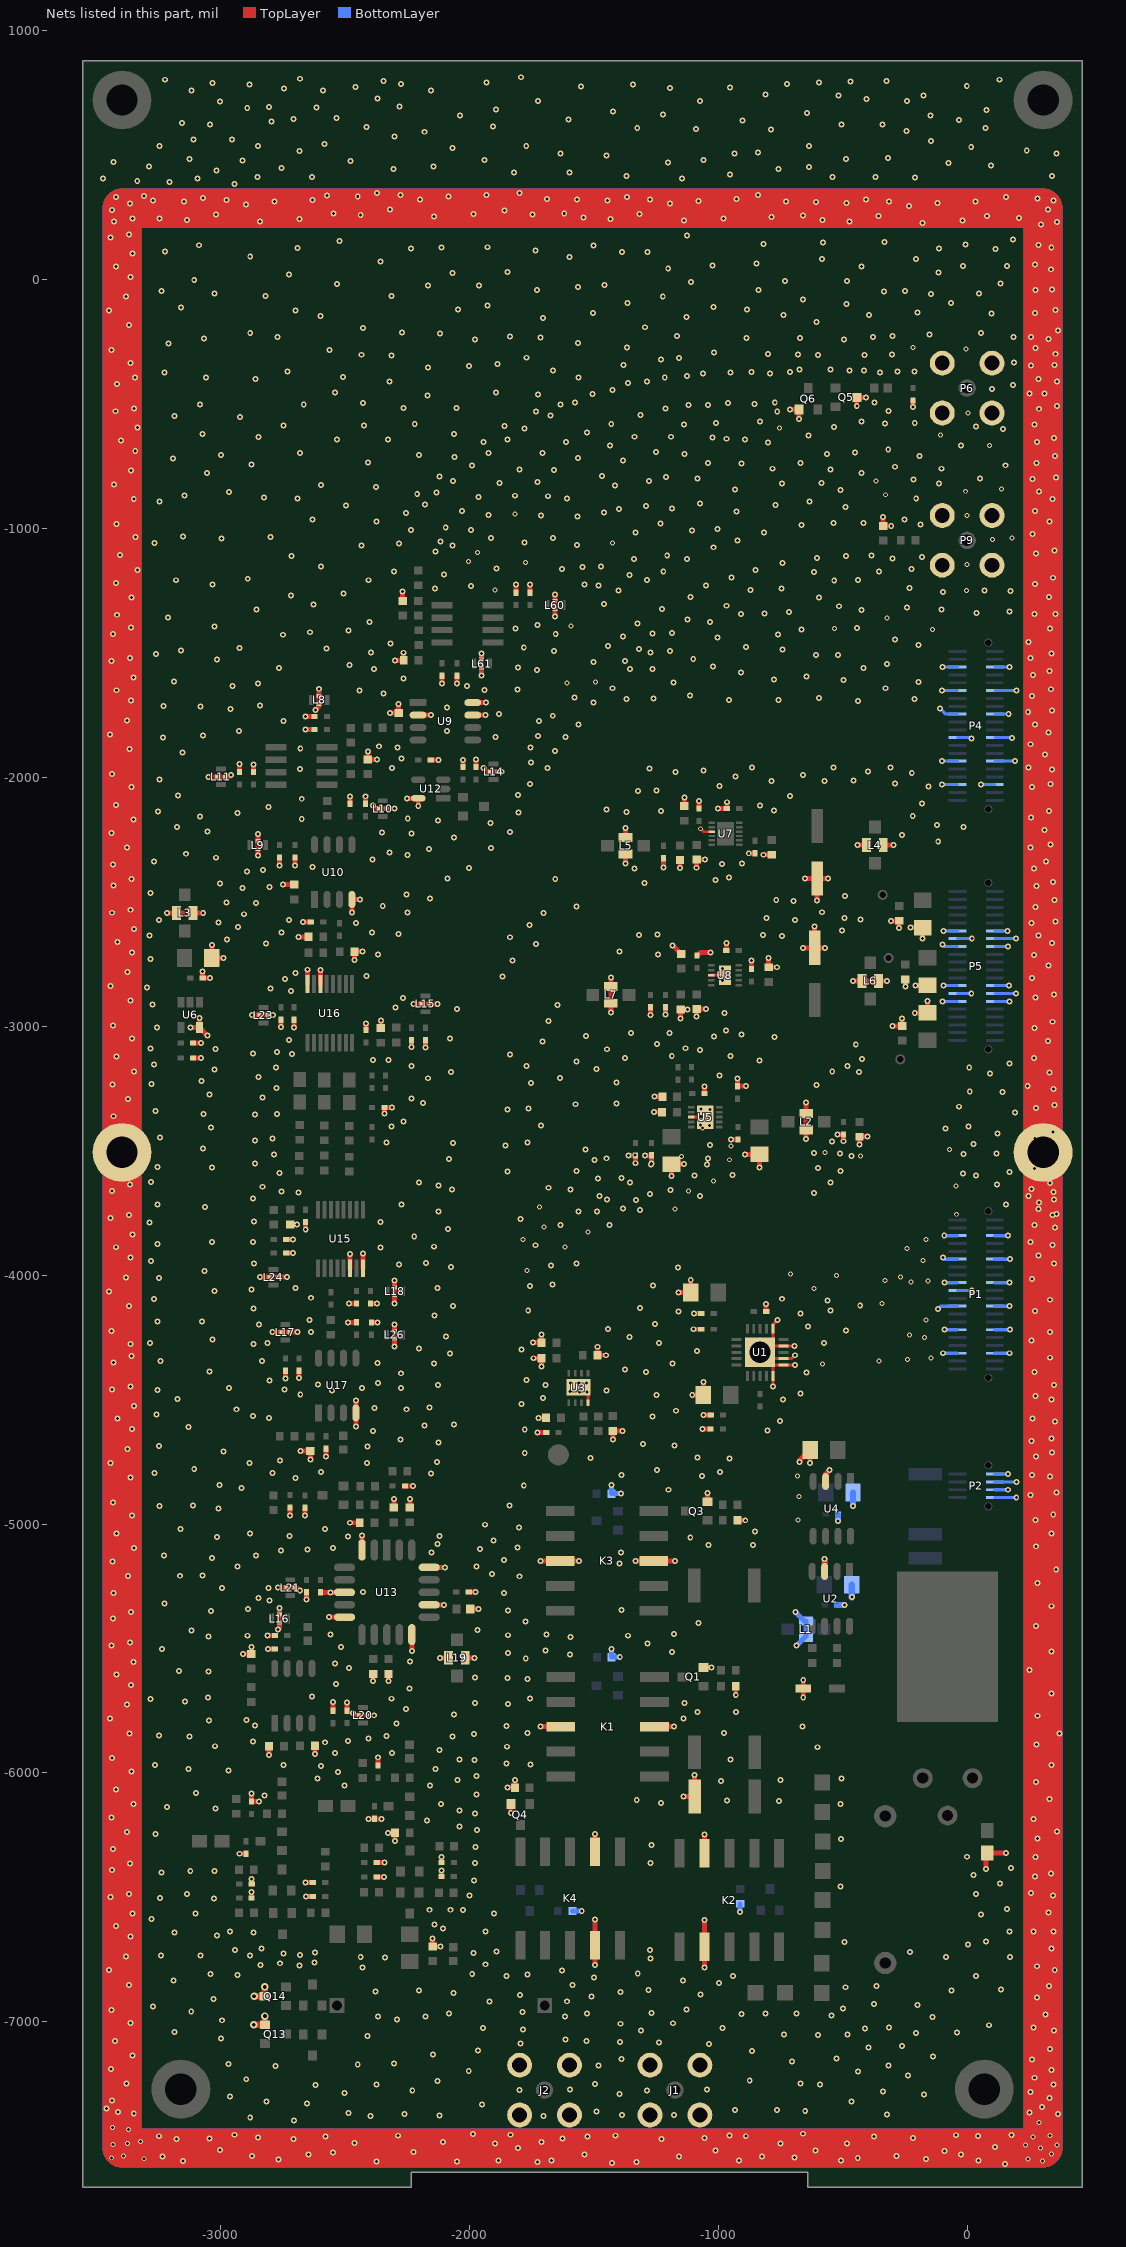
[diagram p0: the nets of this part, all layers, seen from the top]
# Altium PCB MISC109358.PcbDoc (part 4 of 7)
Units mil, origin at the board's own origin, x right, y up, seen from the top; angles counter-clockwise.
Board outline 4015.75 x 8543.31 mil, 4 copper layers (TopLayer, GND, POWER, BottomLayer), stack 33.234 mil thick; 299 components, 170 nets, 998 pads, 2318 vias.

## Via types
v1: diameter 24, hole 12, TopLayer to BottomLayer, 2184 vias
v2: diameter 20, hole 12, TopLayer to BottomLayer, 95 vias
v3: diameter 30, hole 15, TopLayer to BottomLayer, 37 vias
v4: diameter 40, hole 20, TopLayer to BottomLayer, 2 vias

## Nets (pads, with @x,y where several pads share a name; then routed paths per layer and width w, separated by ;. In a path a pad name is that pad's centre, name@x,y a point inside that pad or via, vN(x,y) a via of type N, cw(c..) or ccw(c..) an arc to the next point about the centre after c; other vN are vias at no path point) (continued)
GND: (continued)
  other v1: 152.48,-7571.52 -1427.52,-7566.52 -1726.52,-7562.52 -1328.52,-7562.52 -2373.52,-7560.52 -2050.52,-7560.52 -3150.52,-7559.52 -1883.52,-7557.52 -1669.52,-7557.52 -917.52,-7556.52 -506.52,-7556.52 45.81,-7556.52 -2766.52,-7553.52 -165.52,-7551.52 -439.52,-7547.52 -694.52,-7545.52 -3232.52,-7541.52 -1157.52,-7540.52 -824.52,-7540.52 -2873.52,-7539.52 -284.52,-7539.52 -2645.52,-7532.52 -1537.52,-7532.52 -25.52,-7532.52 -2547.52,-7524.52 -2224.52,-7522.52 -90.56,-7519.52 -1011.52,-7517.52 -608.52,-7516.52 -3002.52,-7515.52 -1805.52,-7507.52 111.04,-7502.52 -750.52,-7489.52 -1897.52,-7488.52 -483.52,-7488.52 -2462.33,-7486.52 -1709.79,-7483.52 -2105.52,-7482.52 -3176.52,-7470.52 -2706.52,-7470.52 -1228.52,-7470.52 -3044.52,-7469.52 -1626.52,-7469.52 -1055.14,-7467.52 -217.52,-7467.52 -2848.52,-7465.52 -373.52,-7461.52 -2579,-7460.52 -1524.52,-7460.52 -3246.63,-7459.52 -889.52,-7459.52 43.48,-7458.52 -2286.52,-7457.52 -1412.52,-7457.52 -954.52,-7456.52 -44.52,-7455.52 177.48,-7454.52 -2944.52,-7453.52 -1834.52,-7453.52 -1984.52,-7450.52 -659.52,-7449.52 -2705.52,-7396.52 -2880.52,-7383.52 -1702,-7378 -2397.52,-7377.52 -2119.52,-7375.52 -1178,-7375 -1387.52,-7373.52 -322.52,-7372.52 365.48,-7370.52 -2261.52,-7369.52 -3348.52,-7367.52 -2485.52,-7365.52 250.48,-7363.52 -3412.52,-7361.52 -1489.9,-7359.52 -650.52,-7358.52 -764.52,-7354.52 -932.52,-7353.52 -3458.52,-7348.52 300.48,-7342.52 -1948.52,-7332.52 -2651.52,-7327.52 -2815.52,-7320.52 -464.52,-7320.52 -3435.52,-7316.21 331.48,-7305.52 -2961.52,-7300.52 -172.52,-7291.52 -1397.52,-7289.52 -2502.52,-7285.52 255.48,-7282.52 -338.52,-7280.52 -2229.52,-7276.52 -1286,-7276 -1798,-7274 -1595,-7272 -1045,-7272 -2618.52,-7253.52 346.48,-7252.52 -2373.52,-7251.52 -591.52,-7251.52 -1494.52,-7249.01 -3378.52,-7247.52 -669.31,-7247.52 -2128.52,-7238.52 -873.52,-7235.52 -2896.52,-7230.52 270.48,-7224.52 -238,-7216 -438,-7200 -2002.52,-7196.52 339.48,-7192.52 -3440.52,-7189.52 -2779.52,-7177.52 -1481.52,-7174.52 -316.52,-7174.52 -2448.52,-7171.52 -2967.52,-7169.52 -2302.99,-7166.52 -704.52,-7159.52 260.48,-7151.52 -1389.52,-7148.52 -524.52,-7146.52 -136.52,-7138.52 -3353.52,-7135.52 -2146.52,-7131.52 -864.52,-7116.52 -1964.52,-7115.52 333.48,-7109.52 -396,-7103 -262,-7096 -1037.52,-7089.52 -1795.02,-7087.52 -1238.06,-7082.52 -1394.52,-7080.52 -3423.52,-7076.52 -1528.52,-7076.52 -1614.52,-7071.52 -2998.52,-7066.52 -2408.6,-7057.52 -598.52,-7052.52 -736.52,-7051.52 -480.52,-7050.52 -205.52,-7044.52 -40.52,-7042.52 -3185.52,-7040.52 -1310.52,-7035.52 349.48,-7035.52 -1783.71,-7031.52 -409.52,-7027.52 -1944.52,-7025.52 -983.52,-7024.52 267.48,-7023.52 -313.83,-7022.52 87.48,-7013.52 -1392.52,-7007.52 -1182.52,-7005.52 -3361.52,-7004.52 -2993.52,-6993.52 -2291.52,-6989.52 -138.52,-6979.52 -2368.04,-6978.52 -2175.52,-6978.52 -1616.52,-6978.52 -544.52,-6974.52 315.48,-6969.52 -907.52,-6968.52 -686.52,-6966.52 -2081.21,-6965.52 -1527.52,-6965.52 -810.52,-6965.52 -1268.4,-6963.52 -1787.52,-6960.52 -3117.52,-6958.52 -3438.52,-6951.52 -1127.82,-6949.52 -498.52,-6946.17 -3271.52,-6937.52 -199.52,-6931.52 -374.52,-6928.52 -1919.52,-6917.52 -1608.09,-6917.18 -3028.52,-6908.52 281.48,-6901.52 -1508.52,-6897.52 -1797.52,-6891.52 -1070.52,-6889.52 -2063.52,-6884.52 -1393.52,-6880.52 -2377.13,-6877.52 -62.52,-6874.52 -2202.52,-6873.52 -1280.52,-6872.52 136.5,-6869.52 -488.52,-6860.9 329.48,-6856.52 -364.52,-6855.52 -3368.52,-6851.52 -1585.52,-6851.52 -997.52,-6843.52 -3188.52,-6834.52 -1141.52,-6833.52 -1499.52,-6822.52 -1851.52,-6815.52 -941.52,-6815.52 35.48,-6815.52 -2931.52,-6811.52 -1767.35,-6809.47 -3040.52,-6808.52 -1988.52,-6807.95 -1323.52,-6805.52 -1628.52,-6794.52 -3447.52,-6792.52 352,-6791 -2429.52,-6781.52 280.48,-6776.52 -2682,-6773.52 -2839.52,-6771.46 -1935.52,-6768.52 -2761.83,-6764.49 -2622,-6760.52 -1271.52,-6745.52 -2338.64,-6740.52 -2436.52,-6739.52 -85.52,-6739.52 172.48,-6739.52 -3379.52,-6736.52 -3238.52,-6732.52 -3080.52,-6732.52 -2881.52,-6732.52 -2681.52,-6731.52 -2747.52,-6725.52 -1982.52,-6723.52 -2620.52,-6720.52 -230.52,-6719.52 -1890.52,-6716.52 -2941.52,-6712.12 -1274,-6710.52 338.48,-6705.7 -2836.02,-6704.52 3,-6689 -492.52,-6678.52 76.48,-6676.91 -3362.52,-6657.52 -3014.52,-6653.79 -2867.52,-6641.52 -3185.52,-6640.52 170,-6637 -2962.52,-6636.52 -1934.52,-6636.52 267.48,-6636.52 347,-6636 -2106.6,-6624.21 -3420.52,-6615.52 -2140.04,-6608.52 -3277.52,-6586.52 56,-6569 -3353.52,-6564.52 -3100.52,-6564.52 -1900.52,-6564.67 326.48,-6560.52 -2026.52,-6550.52 -2160.52,-6549.52 -2075.52,-6549.52 159.48,-6546.52 -3026.92,-6503.52 -3242.52,-6501.52 -3441.52,-6498.52 345,-6492 -1999.71,-6491.52 -3367.52,-6486.52 35.48,-6486.52 -3134.52,-6485.52 257.48,-6481.52 -509.52,-6455.52 132.48,-6443.52 -1980.52,-6432.52 273,-6415 25,-6409 336.48,-6403.52 -3237.52,-6400.52 -3121.52,-6393.98 -3024.52,-6393.98 -3435.52,-6389.52 177,-6381 -3363.52,-6363.52 -1976.52,-6362.4 -1273,-6361 274.48,-6337.52 -0.52,-6336.52 -3432.52,-6305.21 -1974.52,-6296.52 -1268,-6290 -506.52,-6264.52 282,-6263 -3260.52,-6244.46 -3375.52,-6236.52 362,-6236 -1969.23,-6228.52 -2040.52,-6214.52 -2169.52,-6191.7 267,-6185 -3437.52,-6178.52 -1976.52,-6162.52 -2040.52,-6150.52 -3020.39,-6143.5 -3214.52,-6137.52 -509.52,-6125.52 -3350.52,-6124.52 -2113.52,-6124.52 -1230.52,-6120.52 -756.52,-6112.52 -965.52,-6109.9 -1327.52,-6108.52 331,-6105 -2823.66,-6089.52 -1971.08,-6085.52 -3098.52,-6079.52 -3420.52,-6065.52 -2502.52,-6051.16 -2158.52,-6049.52 276,-6037 -988.52,-6032.52 -749.52,-6029.04 -2048.54,-6028.52 -2609.81,-6022.52 -504.52,-6022.52 -1971.08,-6011.51 -2527.52,-5995.36 -3358.52,-5993.52 -2967.52,-5989.61 -3128.52,-5984.52 -2135.93,-5983.52 -2596.3,-5971.52 -2746.52,-5968.17 -3263.52,-5967.19 339,-5967 -1754.52,-5966.52 -1850.52,-5962.52 -1979.01,-5948.52 -2039.52,-5946.52 -951.45,-5946.52 -3435.52,-5940.52 -2539.52,-5919.52 -2310.52,-5919.52 -2120.4,-5908.52 -601.52,-5896.52 -1849.52,-5894.52 -3021.52,-5892.52 278,-5885 -2579.95,-5876.52 -2868.52,-5872.52 -2487.52,-5871.52 -2404.83,-5860.63 -3123.77,-5852.52 -2068.52,-5852.52 -2333.33,-5851.52 -3247.52,-5849.52 -1980.52,-5842.52 372,-5842 -3365.52,-5840.52 -1767.35,-5839.52 -976.12,-5839.49 -661.52,-5812.52 -1850.52,-5811.52 -2861.52,-5809.08 -2293.52,-5800.52 -3045.52,-5788.52 -2895.33,-5786.52 -3444.52,-5781.52 -1139.52,-5781.52 282,-5770 -2062.04,-5764.52 -1083.52,-5755.52 -929.52,-5755.52 -2255.52,-5743.72 -3376.52,-5725.52 -1845.52,-5722.07 -1976.52,-5718.83 -1135.52,-5719.52 -3143.52,-5713.52 -3281.52,-5703.52 -2312.52,-5701.64 -1757.02,-5700.66 -3050.52,-5696.22 -2632.52,-5693.52 339,-5681 -2240,-5660.07 -3359.52,-5646.52 -2536.52,-5642.52 -1766.52,-5622.19 -1847.52,-5618.52 -1976.52,-5616.52 -3417.52,-5604.52 -3048.52,-5592.52 -3166.52,-5590.52 251,-5587 -2483.52,-5577.52 -2540.52,-5560.52 -3350.52,-5553.52 -2237.77,-5552.52 -1773.52,-5539.52 -1595.52,-5524.52 -1844.52,-5518.52 -1185.52,-5514.52 339,-5511 -1693.52,-5507.52 -3234.52,-5501.52 -2515.52,-5493.52 -3438.52,-5487.52 -1284.52,-5480.52 -3364.52,-5475.52 -1594.52,-5453.83 -3047.52,-5451.99 -2891.52,-5448.52 -1363.52,-5448.52 -1844.52,-5446.52 -1689.52,-5444.12 -2558.92,-5443.52 -1176.9,-5441.52 -3116.52,-5427.52 -1967.52,-5425.91 276,-5410 -1080,-5398.14 -1774.52,-5391.52 -3432.52,-5378.52 -3360.52,-5352.52 -3038.52,-5349.52 -1844.52,-5346.52 -1388.52,-5344.52 -2889.52,-5341.04 339,-5330 -3224.52,-5318.52 -2803.52,-5306.21 -2846.52,-5296.52 -3429.52,-5277.21 -1861.52,-5276 -2426.85,-5273.52 -2993.31,-5257.52 -2807.96,-5256.52 282,-5237 -1798.52,-5209.52 -3372.52,-5208.52 -3162.52,-5207.52 -3072.52,-5205.83 -1909.52,-5200.52 358,-5182 -2932.52,-5170.52 -1971.08,-5170.52 -1397.52,-5157.52 -3434.52,-5150.52 -1861.52,-5144.64 -3033.52,-5136.52 -3226.52,-5126.52 -2856.52,-5126.52 -2151.52,-5113.52 -1390.52,-5113.52 -2756.04,-5105.52 -2649.52,-5101.52 -1957.52,-5100.52 -3347.52,-5096.52 -2548.52,-5096.52 -1807.52,-5093.52 276,-5089 -1038.52,-5084.52 -859.52,-5084.52 -2128.52,-5079.52 -1902.52,-5066.52 -1112.52,-5053.52 -3014.52,-5052.52 -2487.52,-5049.52 -2722.52,-5048.52 -2119.86,-5047.52 -2881.52,-5038.52 339,-5038 -3417.52,-5037.52 -852.52,-5028.75 -3160.52,-5020.52 -2579.95,-5020.52 -1800.52,-5013.52 -1937.52,-5002.52 274,-4984 -3355.52,-4965.52 346,-4962 -3007.52,-4936.52 -3244.52,-4926.52 -3109.97,-4924.81 -1838.52,-4924.81 -3432.52,-4912.52 255.48,-4882.52 358.48,-4872.52 -1200.52,-4861.91 -2916.52,-4855.52 -1781.52,-4845.34 -3004.56,-4842.52 -2698.04,-4814.52 -3362.52,-4812.52 333.48,-4808.52 -1065.52,-4806.52 -1388.52,-4802.52 260.48,-4802.52 -2153.52,-4795.91 -3265.52,-4795.52 -2791.59,-4795.52 -2595.52,-4789.83 -992.52,-4790.41 -1245.52,-4783.52 -3105.52,-4778.52 -3441.52,-4753.52 -2883.74,-4753.52 -2411.77,-4753.52 -2130.52,-4750.52 -2761.83,-4743.52 -954.52,-4736.52 -1512.52,-4734.52 -1083.52,-4732.52 277.48,-4728.52 -1777.52,-4714.52 341.48,-4711.52 -2988.83,-4707.52 -3373.52,-4697.52 -2408.83,-4687.75 -3247.52,-4686.52 -1175.52,-4684.52 -1302.52,-4677.52 -2123.52,-4672.15 258.48,-4665.52 -2276.84,-4659.52 338.48,-4656.52 -2386.52,-4626.52 -802.34,-4623.52 -1777.52,-4620.51 -3356.52,-4618.52 -3128.52,-4609.52 -2180.52,-4604.02 -2061.21,-4599.52 352.48,-4588.52 -751.52,-4585.78 -3414.52,-4576.52 262.48,-4575.52 -2805.52,-4574.52 -1263.52,-4567.52 -2868.52,-4565.52 -3256.52,-4559.52 -1169.52,-4544.52 -2936.52,-4538.52 -2252.52,-4538.52 -2380.52,-4533 -2159.52,-4531.52 -3347.52,-4525.52 -1790.52,-4516.52 -739.52,-4499.52 338.48,-4498.52 -3172.26,-4497.52 -1704.52,-4493.52 274.48,-4484.52 -1248.52,-4480.52 -2679.52,-4478.52 -669.52,-4474.52 -1558.52,-4468.52 -1527.52,-4468.52 -1595.46,-4467.52 -2551.52,-4463.52 -1449.52,-4462.52 -3253.52,-4461.52 -3435.52,-4459.52 -2743.5,-4458.52 -2965.37,-4452.52 -2430.52,-4452.52 -2274.06,-4452.52 -3361.52,-4447.52 -1694.26,-4441.52 -2126.52,-4440.52 348.48,-4440.52 -2608.52,-4438.76 -2366.52,-4432.52 -1594.66,-4432.52 -1559.52,-4432.52 -1528.69,-4432.52 -2802.88,-4422.52 -1770.52,-4421.52 -2274.06,-4393.86 -644.52,-4390.52 270.48,-4389.52 -1291,-4388 -3043.52,-4386.56 -1374.52,-4379.52 -2141.52,-4354.52 -1184.52,-4354.56 -2369,-4352.52 -3429.52,-4350.52 -3241.52,-4345.52 -2833.53,-4344.93 332.48,-4331.52 -3357.52,-4324.52 -2078.52,-4314.52 -1085.52,-4304.52 -1791.52,-4297.52 -2201.52,-4294.52 -3361.52,-4276.52 -2867.57,-4275.52 -1238.06,-4272.52 -574.52,-4272.52 -3283.52,-4271.52 -2810.69,-4271.52 258.48,-4261.52 -3031.52,-4258.52 -1356.52,-4248.52 -2093.52,-4246.05 -2636.52,-4228.52 333.48,-4227.52 -3438.52,-4223.52 -486.52,-4221.52 -1442.39,-4216.52 -639.52,-4205.52 -2844.52,-4198.52 -1255,-4195 -3253.52,-4185.52 -3074.52,-4185.52 -2641.52,-4179.41 -2140.52,-4161 -669.52,-4153.52 -1160.52,-4146.57 272.48,-4143.52 -1763.52,-4142.52 -549.52,-4142.52 -2866.52,-4133.52 -1313.52,-4132.52 -2066.52,-4124.46 -3368.52,-4123.52 -429.52,-4121.52 -561.93,-4101.52 332.48,-4098.52 -3267.52,-4095.52 -744.52,-4094.52 -2635.52,-4090.52 -3447.52,-4064.52 -3023.52,-4063.07 -2874.62,-4056.52 -2127.52,-4051.52 -2699.52,-4050.52 -1756.52,-4042.94 -1261.52,-4040.52 -1666.52,-4037.52 260.48,-4014.52 -3247.52,-4011.52 -3379.52,-4008.52 -3064.52,-3983.52 -1162.52,-3969.52 -2073.52,-3966.52 -1671.52,-3960.52 -2282.52,-3956.52 -2865.52,-3952.52 -1569.4,-3952.52 349.48,-3952.52 -2174.52,-3950.52 -3278.52,-3943.52 -3362.52,-3929.52 287.48,-3921.12 -2357.52,-3888.52 -3420.52,-3887.52 -2141.52,-3885.52 -1733.52,-3879.52 343.48,-3878.52 -3253.52,-3874.52 -3034.52,-3866.52 -2869.52,-3866.52 255.48,-3866.52 -2221.52,-3844.52 -3353.52,-3836.52 -2085.52,-3814.52 352.48,-3807.52 -1633.06,-3798.52 -1436.52,-3798.52 270.48,-3798.52 -3284.52,-3788.52 -2356.52,-3786.52 -2865.52,-3783.95 -1795.02,-3773.52 -3441.52,-3770.52 -3367.52,-3758.52 343.48,-3757.52 358.48,-3753.52 -2124.52,-3743.52 -1562.1,-3743.52 -1487,-3743 -1314.52,-3737.52 287.48,-3734.52 -1382,-3731 -3061.52,-3726.52 155.48,-3716.52 -3253.52,-3715.52 -2272.52,-3715.52 289.48,-3708.29 -1330.52,-3697.52 -1446.52,-3696.52 349.48,-3694.78 -2869.52,-3691.64 -1476.52,-3682.52 246.48,-3682.52 -1073,-3681 -1274,-3673 -615,-3670 -2686.52,-3668.52 346.48,-3665.52 -2754.52,-3663.52 -3435.52,-3661.52 -1192.52,-3657.52 -2070.52,-3655.52 -1594,-3655 258.48,-3653.52 -1682.52,-3648.52 -2831.52,-3644.47 -2124.52,-3639.52 -3363.52,-3635.52 119.48,-3635.52 333.48,-3628.52 -549,-3627 -2201.52,-3626.52 -1354.52,-3626.52 -3278.52,-3625.52 -1484,-3612 -1388.52,-3609.52 -1095.74,-3599.52 35.48,-3599.52 -942.52,-3596.52 -16.52,-3590.52 -2763.52,-3588.52 -1846,-3584 169.34,-3584.52 -508,-3582 -1569.4,-3580.31 271.48,-3570.52 -599,-3569 -3033.26,-3567.43 -3253.52,-3565.95 -1044.52,-3555.52 -1270.89,-3554.52 -2860.52,-3551.52 -1498.08,-3537.52 -2081.21,-3533.52 -1040.78,-3531.52 -1449,-3530 -464,-3521 -2784.52,-3515.52 -13.99,-3513.52 -511,-3511 118.08,-3510.52 -616,-3508 328.48,-3501.83 -1533,-3494 -3070.52,-3490.52 -1854,-3479 -1032.52,-3477.52 25.48,-3472.52 -2065.52,-3469.52 -2333.33,-3467.52 -1766,-3467 -543.52,-3463.52 -2861.52,-3458.52 -2791.52,-3450.52 273.48,-3450.52 -3243.52,-3446.52 122.48,-3430.52 345.48,-3424.52 -87.52,-3409.52 -3037.31,-3406.52 5.48,-3402.52 -2313.52,-3401.52 -1713,-3399 -1035.38,-3397.52 -1070.52,-3395.52 -2265.09,-3382.52 -1069.52,-3362.52 -1034.52,-3362.52 -3429.52,-3361.21 -2861.52,-3355 -3067.52,-3352.52 -2773.52,-3352.52 191.54,-3345.52 -3260.52,-3340.52 -1846,-3335 -1033.52,-3333.52 -1069.52,-3332.52 -1762,-3331 277.48,-3327.52 -32,-3323 351.48,-3315.52 -1573,-3313 -1408,-3310 -2186.52,-3308.52 -3372.52,-3292.52 -2233.52,-3290.52 -2831.84,-3286.52 -3043.52,-3274.52 142.48,-3264.52 10.48,-3261.52 346.48,-3251.78 -2775.29,-3247.52 243.48,-3239.52 -605,-3235 -3434.52,-3234.52 -3277.52,-3232.52 -1752,-3228 -1408,-3226 -3075.52,-3219.52 -2165.52,-3208.52 -1635,-3208 -2846.52,-3203.52 -995,-3197 92.48,-3189.52 330.48,-3185.52 -435,-3184 -2074.52,-3183.52 -542,-3182 -3347.52,-3180.52 -3024.52,-3172.52 -1489,-3171 8.48,-3165.52 -2777,-3164.52 -1770,-3160 -2233.52,-3159.52 -481.23,-3159.52 -3267.52,-3152.52 169.34,-3148.52 -1569,-3142 -833.52,-3137.06 -2387.52,-3135.52 -2324.52,-3135.52 -423,-3132 -1375,-3127 268.48,-3127.52 -3417.52,-3121.52 -1186.85,-3118.52 -951.45,-3118.52 -1836,-3113 -2712.52,-3110.52 -2869.52,-3109.52 -2773.52,-3102.52 -1072.52,-3094.52 -1447,-3092 -3020.39,-3090.52 -3281.52,-3088.52 -1131,-3088 -447.52,-3072.52 -1246,-3070 -1706,-3060 325.48,-3058.83 -2725.52,-3054.52 -3355.52,-3049.52 -2077.52,-3048.52 -773.52,-3043.52 -1018.04,-3041.52 -1532,-3039 -907.52,-3033.52 -1351,-3027 -1195.52,-3027.52 -968,-3016 270.48,-3007.52 -3254.52,-3004.77 -3432.52,-2996.52 342.48,-2981.52 -1682,-2979 -975.52,-2946.52 -2049.39,-2929.52 -2296.52,-2923.52 -1645,-2914 -3273.52,-2912.52 -3362.52,-2896.52 -2266.52,-2885.52 274.48,-2884.52 348.48,-2872.52 -2716.52,-2857.52 -2799.52,-2847.52 -3294.52,-2844.52 -3441.52,-2837.52 -983.52,-2815.52 -2740.52,-2809.52 260.48,-2806.52 -1867,-2800 -2413.52,-2798.52 -963.52,-2793.52 -2698.52,-2786.52 -3373.52,-2781.52 -983.52,-2768.52 327.48,-2755.52 -1826,-2735 -3281.52,-2729.53 269.48,-2713.52 -1242,-2712 -2366.52,-2710.52 -3356.52,-2702.52 -1396,-2700 -1733,-2669 -2817.52,-2666.4 340.48,-2665.52 -3414.52,-2660.52 -2974.21,-2651.52 -1836,-2642 -743.52,-2636.52 -3285.52,-2634.52 286.48,-2634.52 -1318,-2632 -819.52,-2632.52 -1244,-2630 -2285.52,-2628.52 -2754.52,-2622.52 -2390.96,-2622.35 -503.52,-2614.52 -3347.52,-2609.52 -2930.52,-2601.52 -1758,-2593 -2455.12,-2583.88 259.48,-2584.52 -3008.39,-2581.83 354.48,-2578.52 -3247.52,-2573.52 -692.52,-2573.52 -2724.52,-2572.52 -428.52,-2570.52 -806.52,-2565.52 -493.52,-2564.52 -2904.65,-2549.52 -1702,-2544 -3435.52,-2543.52 -2248.52,-2542.52 -582.52,-2541.52 -3361.52,-2531.52 -1569,-2519 275.48,-2519.52 -2348.08,-2516.52 -2857.52,-2503.57 -2975.52,-2502.52 -698.52,-2496.52 -767,-2492 350.48,-2492.52 -2158.9,-2485.52 -491.52,-2476.52 -2253.52,-2470.52 -3281.52,-2464.52 -2911.52,-2444.97 -2802.88,-2440.52 278.48,-2435.52 -3429.52,-2434.52 -3001.52,-2425.52 -1295.52,-2424.52 345.48,-2419.52 -1012,-2412 -3357.52,-2408.52 -1655,-2408 -2088.52,-2405.52 -955.94,-2401.52 -2893.35,-2377.48 -2829.23,-2372.39 268.48,-2366.52 -1336,-2365 -2002.1,-2363.52 -2630.52,-2360.52 -3432.52,-2350.21 -984.52,-2347.52 -903.7,-2346.52 -3267.52,-2338.52 316.48,-2338.52 -2389.8,-2329.78 -3018.52,-2322.52 -2249.52,-2312.19 -3139.52,-2306.52 -2320.52,-2301.52 -2161.46,-2287.27 -1912.52,-2283.52 -3375.52,-2281.52 254.48,-2280.52 335.48,-2269.49 -116.12,-2256.52 -2061.21,-2240.52 -261.52,-2230.52 -2233.52,-2225.52 -3437.52,-2223.52 -2350.52,-2221.52 -1836.52,-2218.52 -3052.86,-2217.52 311.48,-2211.83 -3175.52,-2199.38 -13.99,-2198.52 -122.02,-2191.52 -1914.39,-2182.52 -2126.83,-2172.52 -3350.52,-2169.52 -2673.52,-2166.52 -2247.65,-2164.52 256.48,-2160.52 -3081.52,-2157.52 -218.52,-2154.52 -2932.52,-2142.52 -1803.52,-2140.4 -1368.52,-2139.52 -3251.52,-2137.52 -1229.52,-2134.52 328.48,-2134.52 -776.52,-2132.52 -1450,-2128 -2807.52,-2119.52 -831.82,-2112.52 -3420.52,-2110.52 -181.52,-2104.52 -2673.52,-2085.52 -711.52,-2073.52 -3170.52,-2072.52 -1805,-2071 -1322,-2054 -1248.39,-2051.52 -3358.52,-2038.52 260.48,-2037.52 -154.52,-2036.52 -994.12,-2033.36 -1756,-2027 334.48,-2025.52 -290.52,-2023.52 -572.52,-2014.52 -786.52,-2013.52 -456.72,-2012.52 -3244.52,-2007.52 -931,-1996 -658.76,-1989.52 -3435.52,-1985.52 -222.52,-1982.52 -1172.52,-1978.52 -398.52,-1975.52 -1059.52,-1972.52 341.48,-1968.52 -2680.52,-1966.01 -1277,-1964 -2311.52,-1961.52 -1687,-1961 -863.52,-1960.69 -536.52,-1960.69 -307.78,-1960.69 246.48,-1959.52 -1752,-1940 -2272.52,-1924.52 313.48,-1908.52 -3152.52,-1900.52 -1656,-1893 -3365.52,-1885.52 -2679.52,-1883.52 -1754,-1880 -2288.52,-1879.52 -2362.52,-1874.57 255.48,-1866.52 -3230.52,-1838.52 -1614,-1838 -1895.52,-1836.5 -1725,-1833 -3069.52,-1831.52 -3444.52,-1826.52 326.48,-1818.52 -2089.92,-1813.52 -2926.52,-1812.52 -1562.1,-1787.52 272.48,-1787.52 -2747.52,-1773.52 -1721,-1773 -3376.52,-1770.52 -1665,-1752 -1880.52,-1745.52 245.48,-1737.52 340.48,-1731.52 -2960.52,-1725.52 -2089.92,-1718.52 -3079.52,-1714.52 -3228.52,-1712.52 -2841.52,-1710.52 -1500.52,-1699.52 -438.52,-1692.52 -3359.52,-1691.52 -956.52,-1688.52 -758.52,-1688.52 -1368,-1685 -211.52,-1685.52 -1259.52,-1682.52 -594.52,-1681.31 -1577,-1678 261.48,-1672.52 -1112.76,-1671.52 -2345.52,-1663.52 -2441.52,-1650.52 -3417.52,-1649.52 -1938.52,-1648.52 -1806.21,-1646.52 336.48,-1645.52 -1424.52,-1641.52 -327.52,-1641.52 -2010.52,-1632.95 -2951.52,-1631.52 -2848.52,-1621.52 -1179.76,-1618.52 -195.52,-1615.52 -3186.48,-1613.52 -496.52,-1607.52 -776.52,-1605.52 -2264.52,-1602.52 -3350.52,-1598.52 -644.52,-1594.52 264.48,-1588.52 -908.69,-1578.52 331.48,-1572.52 -1727.36,-1567.52 -1354.52,-1564.52 -1265,-1564 -2384.02,-1563.52 -2764.52,-1560.52 -415.52,-1560.52 -1804.52,-1557.52 -1020.52,-1554.52 -2480.81,-1548.52 -322.52,-1544.52 -1501.52,-1535.52 -3438.52,-1532.52 -1375,-1532 -3014.52,-1525.52 -1100.52,-1523.52 -3364.52,-1520.52 254.48,-1519.52 -607.52,-1507.52 -519.52,-1507.52 -3258.52,-1503.52 338.48,-1502.52 -1272.52,-1498.52 -2395.95,-1497.52 -1659.52,-1492.52 -1194,-1491 -3159.3,-1489.52 -741.52,-1486.52 -1318,-1483 -2574.52,-1482.52 -2923.52,-1480.52 -1781.52,-1478.52 -888.52,-1476.52 -1443,-1471 -194.52,-1468.52 -2316.52,-1461.52 246.48,-1455.52 -290.52,-1445.52 -1002.52,-1438.52 -1383,-1433 -2748.21,-1426.52 -759.52,-1425.52 -1653,-1424 -3432.52,-1423.52 -1264,-1421 -1185.52,-1419.52 -2639.52,-1416.52 -2485.52,-1409.52 -665.52,-1405.52 -1814.52,-1401.52 333.48,-1401.52 -442.52,-1398.52 -3360.52,-1397.52 -3023.52,-1392.52 -1726.52,-1387.52 -1325,-1382 -1034,-1376 -2401.52,-1374.71 -1123,-1365 -3210.52,-1358 -3415.52,-1346.21 -908.69,-1343.52 271.48,-1343.52 355.48,-1343.52 -814,-1341 38.48,-1338.52 -716.52,-1334.52 170.48,-1333.52 -425,-1328 -2855.52,-1324.52 -103.52,-1324.52 -1227,-1323 -241.52,-1316.52 -514,-1312 -966,-1310 -2626.52,-1304.52 -1459.52,-1302.52 -3358.52,-1277.52 -596,-1277 328.48,-1274.83 -1111,-1274 -2716.52,-1269.52 -2506.52,-1261.52 -97.52,-1255.52 174.48,-1250.52 -1400,-1248 69.53,-1248.52 -870,-1246 -2138.52,-1240.52 -746,-1240 -232.52,-1238.52 -1993.52,-1230.52 -1482,-1228 -1050,-1228 -3032.52,-1225.52 -1538,-1225 273.48,-1223.52 -3420.52,-1219.52 -534,-1209 -3179.52,-1207.52 -2404.52,-1207.52 -1287,-1207 -438,-1207 -2890.52,-1201.52 -947,-1197 345.48,-1197.52 -1357,-1186 -2101.95,-1184.52 -615,-1174 -1221,-1172 -2303.52,-1171.52 -354.52,-1171.52 -851,-1167 -3333.52,-1165.52 -223,-1162 -1627.52,-1161.52 -1891.52,-1159.52 -1545.16,-1154.52 -2595.52,-1152.52 -1471.52,-1151.52 -742,-1139 -1338,-1123 -1125,-1123 -300.52,-1120.52 -603,-1119 -181.52,-1114.52 -487,-1111 -2713.88,-1110.52 -1205,-1108 -384,-1108 -3403.52,-1106.52 277.48,-1100.52 -2135.93,-1092.52 351.48,-1088.52 -1020,-1075 -2432.52,-1068.52 -2067.52,-1068.52 -1567.52,-1066.52 -2283.52,-1059.52 -3264.52,-1057.52 -1778.52,-1056.52 -2116,-1051 -923,-1047 -2995.52,-1039.52 -1912.52,-1038.52 -1663.52,-1038.52 -3341.52,-1034.52 -2799.52,-1033.52 -3151.52,-1031.52 263.48,-1022.52 -1332,-1016 -816,-1016 -1106,-1007 -2234,-1006 -1993,-1006 -1003,-1001 -2095,-995 -666,-985 -188,-983 -3418.52,-981.52 -1232,-979 -537,-977 -417,-977 -2373.52,-971.52 330.48,-971.52 -252.09,-964.18 -2629.52,-962.52 -1566,-952 -1712.52,-946.52 -1924,-945 -2255.52,-936.52 -1459.52,-935.52 -926.31,-930.52 -2029,-929 272.48,-929.52 -1398,-922 -1186,-919 -489,-913 -1291,-909 -2495.52,-906.52 -769.52,-904.52 -2179,-903 -1073.52,-899.52 -633,-892 -3244.52,-890.52 -3348.52,-881.52 343.48,-881.52 -1607,-880 -2690.52,-878.83 -204.52,-879.52 -2824.52,-875.52 -1963,-873 -1684,-870 -1816,-868 -3145.52,-866.52 -2209.52,-860.52 -2132,-855 -2965.52,-853.52 289.48,-850.52 -508.52,-845.52 -933.52,-843.52 -2375.52,-833.52 -1415,-826 -2596.52,-824.52 -3427.52,-822.52 -744,-818 -113,-818 -1879,-816 -585.52,-816.52 -1726,-813 -1279,-809 -2066,-808 -215,-802 262.48,-800.52 -1082.52,-799.52 51.48,-799.52 357.48,-794.52 -1210.52,-793.52 -2120,-790 -1467,-789 -425,-777 -3054.52,-776.52 -3359.52,-766.52 -1660,-764 -1798,-763 -549,-763 -781.52,-759.52 -102.52,-759.52 -289.52,-751.52 -1989,-746 153.48,-745.52 -2875.04,-742.52 -1041,-737 -906.52,-737.52 -669.31,-735.52 278.48,-735.52 -2407.52,-733.52 -1382,-727 -3191.52,-718.52 -1563,-716 -2060,-713 -190.52,-708.52 353.48,-708.52 -2998.04,-704.52 -2202.52,-704.52 -1136.52,-700.52 -562.52,-700.52 -1923,-697 -1707,-697 -2680.08,-696.52 -451.52,-694.52 -1250,-693 -3342.52,-687.52 -317,-683 -1435,-667 -25.52,-666.52 -800,-655 -1612,-653 -1943,-652 281.48,-651.52 -3400.52,-645.52 -2531.52,-642.52 -2327,-642.52 -1847,-642 -892,-642 -967,-639 348.48,-635.52 -1023,-634 -2846.52,-631.52 -1337,-631 -1190,-631 -636.52,-626.52 -3071.52,-620.52 -2062.52,-620.52 -1528,-614 144.48,-600.52 -1779,-597 -3333.52,-594.52 -535.52,-592.52 36.48,-589.52 -1859,-588 -2747.52,-586.52 -2423.52,-586.52 -1137,-582 271.48,-582.52 -2219.52,-580.52 -1430,-579 -329.52,-578.52 -210.52,-576.52 -1010,-575 -832,-570 -423.52,-568.89 -2921.52,-551.52 -3185.52,-548.52 -1675,-546 -1313,-544 -1733,-530 -763,-529 -3421.52,-528.52 -315.52,-526.89 288.48,-518.5 -1212,-517 -3347.52,-516.52 -2265.09,-514.52 -2052.52,-514.52 361.48,-506.52 -1120,-503 -1041,-503 -1633,-502 -3082.52,-500.52 -2665.52,-500.52 -854,-500 -960,-496 -2426.85,-494.52 -372,-494 -1575,-493 -773,-493 -2167.52,-464.52 -1725,-461 -1505,-459 311.48,-457.52 251.48,-456.34 -2539.52,-452.52 -1892.52,-452.52 -1425,-444 100,-440 183.48,-423.46 -3415.52,-419.52 -1363,-415 -2321.52,-409.81 -1287,-409 360.48,-408.52 -2858.52,-398.52 287.48,-398.52 -3343.52,-393.52 -1561,-393 -1215,-393 -3057.52,-392.52 -2508.52,-390.52 -1125,-387 -1061,-376 -792,-376 -3224.52,-373.52 -950,-372 -351,-372 -866,-370 -711,-370 -2730.52,-369.52 -211.52,-368.89 -279.52,-367.89 -1663.52,-365.52 -414.52,-364.89 -472,-364 -674.52,-360.89 -548.52,-360.89 -2165.52,-352.52 -2001.52,-346.52 257.48,-344.52 -1380,-343 350.48,-343.52 -1887,-339 -3361.52,-335.52 188.48,-332.52 -1231,-321 -1157,-314 -1770.52,-313.52 -2312.52,-304.52 -599,-303 -412,-303